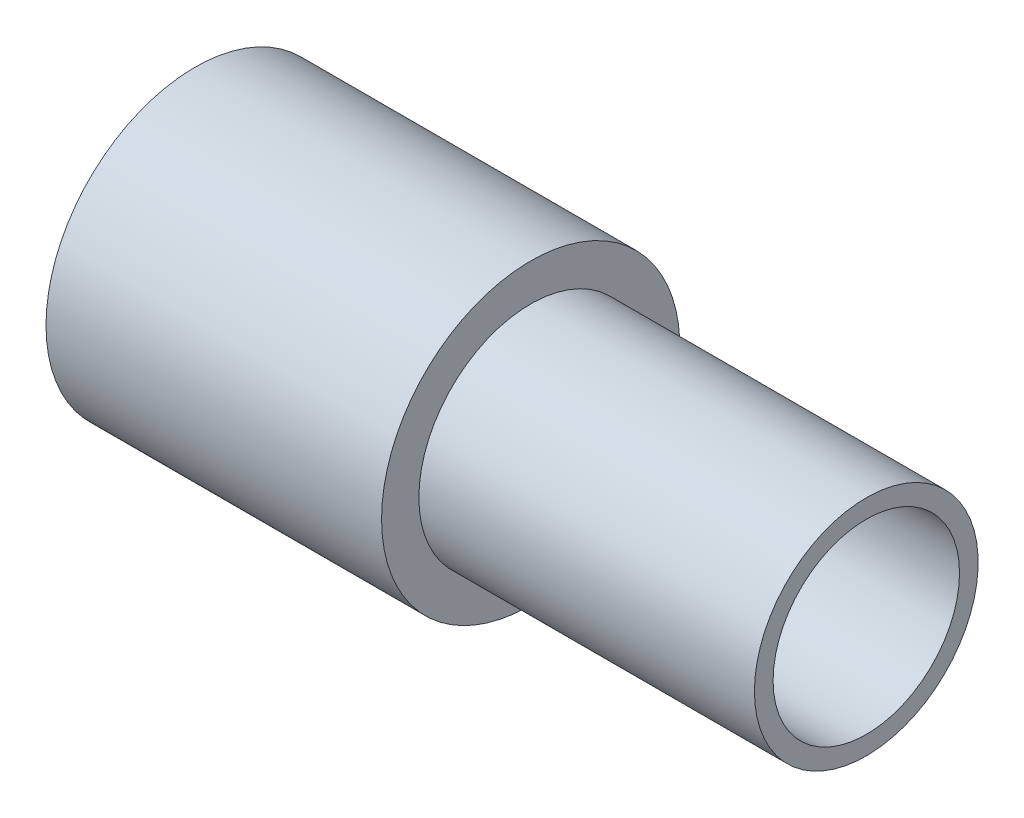
from build123d import *

# Parameters (mm, degrees)
CUT_EXTRUDE_1_REACH = 96.34
SKETCH_2_R          = 12.5


with BuildPart() as part:
    # 草图1 → 旋转1 (revolve)
    with BuildSketch(Plane.XY, mode=Mode.PRIVATE) as revolve_1_sk:
        Polygon((0, 0), (0, 20), (45, 20), (45, 15), (90, 15), (90, 0), align=None)
    revolve(revolve_1_sk.sketch.rotate(Axis((-36.553846154, 0, 0), (1, 0, 0)), 90), axis=Axis((-36.553846154, 0, 0), (1, 0, 0)))

    # 草图2 → 切除-拉伸1 (cut, up to next)
    with BuildSketch(Plane(origin=(90, 0, 0), x_dir=(0, 0, -1), z_dir=(1, 0, 0)), mode=Mode.PRIVATE) as cut_extrude_1_sk1:
        Circle(SKETCH_2_R)
    cut_extrude_1_tool1 = extrude(cut_extrude_1_sk1.sketch, amount=-CUT_EXTRUDE_1_REACH, mode=Mode.PRIVATE) & part.part
    add(cut_extrude_1_tool1.solids().sort_by_distance((90, 0, 0))[0], mode=Mode.SUBTRACT)


solid = part.part
